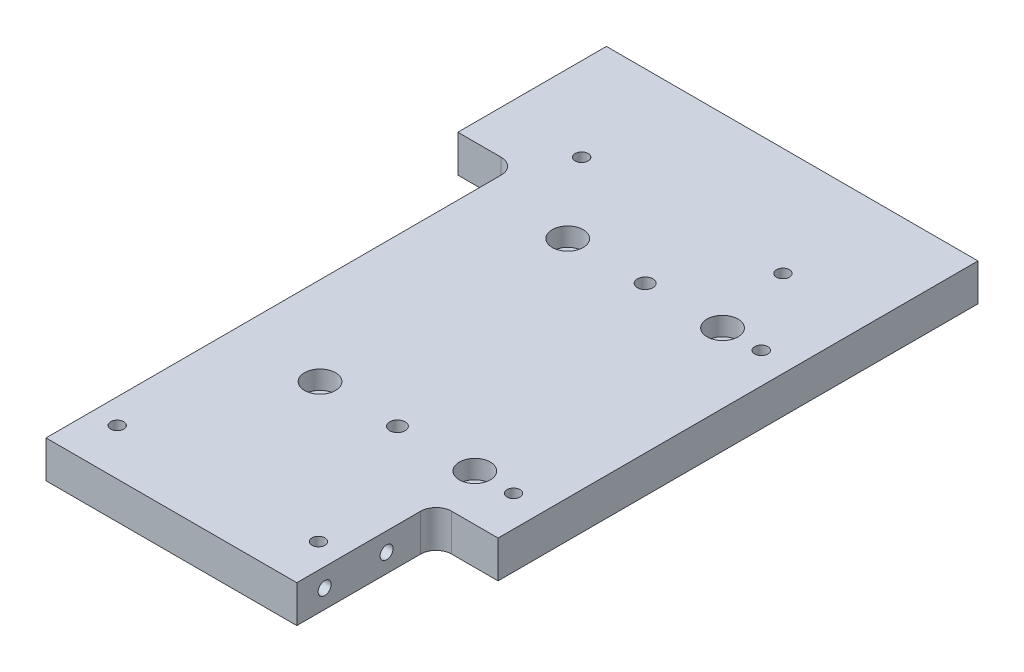
SolidWorks part; units mm, degrees
material "45#"
ref_plane "Front Plane" through (0, 0, 0) normal (0, 0, 1) x (1, 0, 0)
ref_plane "Top Plane" through (0, 0, 0) normal (0, 1, 0) x (1, 0, 0)
ref_plane "Right Plane" through (0, 0, 0) normal (1, 0, 0) x (0, 0, -1)
sketch "Sketch1" plane through (0, 0, 0) normal (0, 1, 0) x (1, 0, 0)
  line L0 (60, 100) -> (-60, -100) construction
  line L1 (-60, 100) -> (60, 100)
  line L2 (-60, 100) -> (-60, -100)
  line L3 (-60, -100) -> (60, -100)
  line L4 (60, 100) -> (60, -100)
  dimension "D1" = 120
  dimension "D2" = 200
extrude "Extrude1" add sketch "Sketch1" along normal mid plane 12
sketch "Sketch2" plane through (0, 6, 0) normal (0, 1, 0) x (1, 0, 0)
  line L1 (300, 85) -> (60, 85)
  line L2 (300, 85) -> (300, -70)
  line L3 (300, -70) -> (60, -70)
  line L4 (60, 85) -> (60, -70)
  line L5 (60, 100) -> (-60, 100) construction
  line L6 (-60, -100) -> (60, -100) construction
  line L7 (60, -100) -> (60, 100) construction
  dimension "D1" = 240
  dimension "D2" = 15
  dimension "D3" = 30
extrude "Extrude2" [suppressed] add sketch "Sketch2" against normal up to vertex
sketch "Sketch3" plane through (0, 6, 0) normal (0, 1, 0) x (1, 0, 0)
  line L1 (-41, 52) -> (-60, 52)
  line L2 (-41, 52) -> (-41, -100)
  line L3 (-41, -100) -> (-60, -100)
  line L4 (-60, 52) -> (-60, -100)
  line L5 (-60, 100) -> (-60, -100) construction
  line L6 (60, 100) -> (-60, 100) construction
  dimension "D1" = 48
  dimension "D2" = 19
extrude "Cut-Extrude1" cut sketch "Sketch3" against normal through all
fillet "Fillet1" radius 5 1 edges at (-41, 0, -52)
sketch "Sketch4" plane through (0, 6, 0) normal (0, 1, 0) x (1, 0, 0)
  line L0 (60, -100) -> (60, 100) construction
  line L1 (60, -55) -> (40, -55)
  line L2 (60, -55) -> (60, -100)
  line L3 (60, -100) -> (40, -100)
  line L4 (40, -55) -> (40, -100)
  line L5 (-41, -100) -> (60, -100) construction
  line L6 (-41, -100) -> (-41, 47) construction
  dimension "D1" = 81
  dimension "D2" = 45
extrude "Cut-Extrude2" cut sketch "Sketch4" against normal through all
sketch "Sketch5" plane through (0, 6, 0) normal (0, 1, 0) x (1, 0, 0)
  point P0 (-12.5, 40)
  point P1 (12.5, 40)
  point P3 (37.5, 40)
  point P7 (-12.5, -40)
  point P8 (12.5, -40)
  point P10 (37.5, -40)
sketch "Sketch6" plane through (0, 6, 0) normal (0, 1, 0) x (1, 0, 0)
  circle A0 centre (12.5, 40) radius 2.5
  circle A1 centre (12.5, -40) radius 2.5
  dimension "D1" = 5
extrude "Cut-Extrude3" cut sketch "Sketch6" against normal through all
hole_wizard "M5 Socket Head Cap Screw Counterbore1" positions "3D Sketch1" profile "Sketch7" counterbore size "M5" standard "ISO" end condition through all
sketch3d "3D Sketch1"
  point P0 (37.5, 6, -40)
  point P3 (-12.5, 6, -40)
  point P6 (-12.5, 6, 40)
  point P9 (37.5, 6, 40)
sketch "Sketch7" plane through (37.5, 6, -40) normal (1, 0, 0) x (0, 0, 1)
  line L0 (0, 0) -> (0, 12)
  line L1 (0, 12) -> (2.75, 12)
  line L3 (2.75, 12) -> (2.75, 6)
  line L4 (2.75, 6) -> (5, 6)
  line L5 (5, 6) -> (5, 0)
  line L7 (5, 0) -> (0, 0)
  line L11 (0, -6.35) -> (0, 107.95) construction
  dimension "貫穿孔直徑" = 5.5
  dimension "貫穿孔深度" = 12
  dimension "柱孔直徑" = 10
  dimension "柱孔深度" = 6
hole_wizard "M5 Tapped Hole1" positions "3D Sketch2" profile "Sketch8" tap size "M5" standard "ISO" end condition through all
sketch3d "3D Sketch2"
  line L0 (32, 6, -65) -> (32, 6, 85) construction
  line L1 (32, 6, 85) -> (-33, 6, 85) construction
  line L2 (-33, 6, 85) -> (-33, 6, -65) construction
  line L3 (-33, 6, -65) -> (32, 6, -65) construction
  line L5 (-41, 6, 100) -> (40, 6, 100) construction
  line L6 (-41, 6, 100) -> (-41, 6, -47) construction
  point P0 (32, 6, 85)
  point P2 (-33, 6, 85)
  point P4 (32, 6, -65)
  point P6 (-33, 6, -65)
  dimension "D1" = 65
  dimension "D2" = 8
  dimension "D3" = 15
  dimension "D4" = 150
sketch "Sketch8" plane through (32, 6, 85) normal (1, 0, 0) x (0, 0, 1)
  line L0 (0, 0) -> (0, 12)
  line L1 (0, 12) -> (2.1, 12)
  line L2 (2.1, 12) -> (2.1, 0)
  line L5 (2.1, 0) -> (0, 0)
  line L11 (0, -6.35) -> (0, 107.95) construction
  dimension "貫穿螺孔鑽直徑" = 4.2
  dimension "貫穿螺孔鑽深度" = 12
cosmetic thread "Cosmetic Thread7" parameters "D2"=5
cosmetic thread "Cosmetic Thread8" parameters "D2"=5
cosmetic thread "Cosmetic Thread9" parameters "D2"=5
cosmetic thread "Cosmetic Thread10" parameters "D2"=5
fillet "Fillet2" radius 5 1 edges at (40, 0, 55)
hole_wizard "M5 Tapped Hole2" positions "3D Sketch3" profile "Sketch9" tap size "M5" standard "ISO"
sketch3d "3D Sketch3"
  line L0 (40, 0, 100) -> (40, 0, 91) construction
  line L1 (40, -6, 100) -> (40, 6, 100) construction
  line L2 (40, 0, 91) -> (40, 0, 71) construction
  point P0 (40, 0, 91)
  point P2 (40, 0, 71)
  dimension "D1" = 9
  dimension "D2" = 20
sketch "Sketch9" plane through (40, 0, 91) normal (0, 1, 0) x (0, 0, -1)
  line L0 (0, 0) -> (0, 13.6618)
  line L1 (0, 13.6618) -> (2.1, 12.4)
  line L2 (2.1, 12.4) -> (2.1, 0)
  line L5 (2.1, 0) -> (0, 0)
  line L10 (0, 13.6618) -> (-2.1, 12.4) construction
  line L11 (0, -6.35) -> (0, 107.95) construction
  dimension "螺孔鑽直徑" = 4.2
  dimension "螺孔鑽深度" = 12.4
  dimension "導頭角度" = 118
cosmetic thread "Cosmetic Thread5" parameters "D1"=10, "D2"=5
cosmetic thread "Cosmetic Thread6" parameters "D1"=10, "D2"=5
hole_wizard "M5 Tapped Hole3" positions "3D Sketch4" profile "Sketch10" tap size "M5" standard "ISO" end condition through all
sketch3d "3D Sketch4"
  line L0 (0, 6, -100) -> (-0.5, 6, 100) construction
  line L1 (60, 6, -100) -> (-60, 6, -100) construction
  line L2 (-41, 6, 100) -> (40, 6, 100) construction
  line L4 (-0.25, 6, 0) -> (80.7527, 6, 0) construction
  line L6 (50, 6, -40) -> (50, 6, 0) construction
  line L7 (50, 6, 0) -> (50, 6, 40) construction
  line L9 (60, 6, 55) -> (60, 6, -100) construction
  point P0 (50, 6, -40)
  point P2 (50, 6, 40)
  dimension "D1" = 80
  dimension "D2" = 10
sketch "Sketch10" plane through (50, 6, -40) normal (1, 0, 0) x (0, 0, 1)
  line L0 (0, 0) -> (0, 12)
  line L1 (0, 12) -> (2.1, 12)
  line L2 (2.1, 12) -> (2.1, 0)
  line L5 (2.1, 0) -> (0, 0)
  line L11 (0, -6.35) -> (0, 107.95) construction
  dimension "貫穿螺孔鑽直徑" = 4.2
  dimension "貫穿螺孔鑽深度" = 12
cosmetic thread "Cosmetic Thread11" parameters "D2"=5
cosmetic thread "Cosmetic Thread12" parameters "D2"=5
